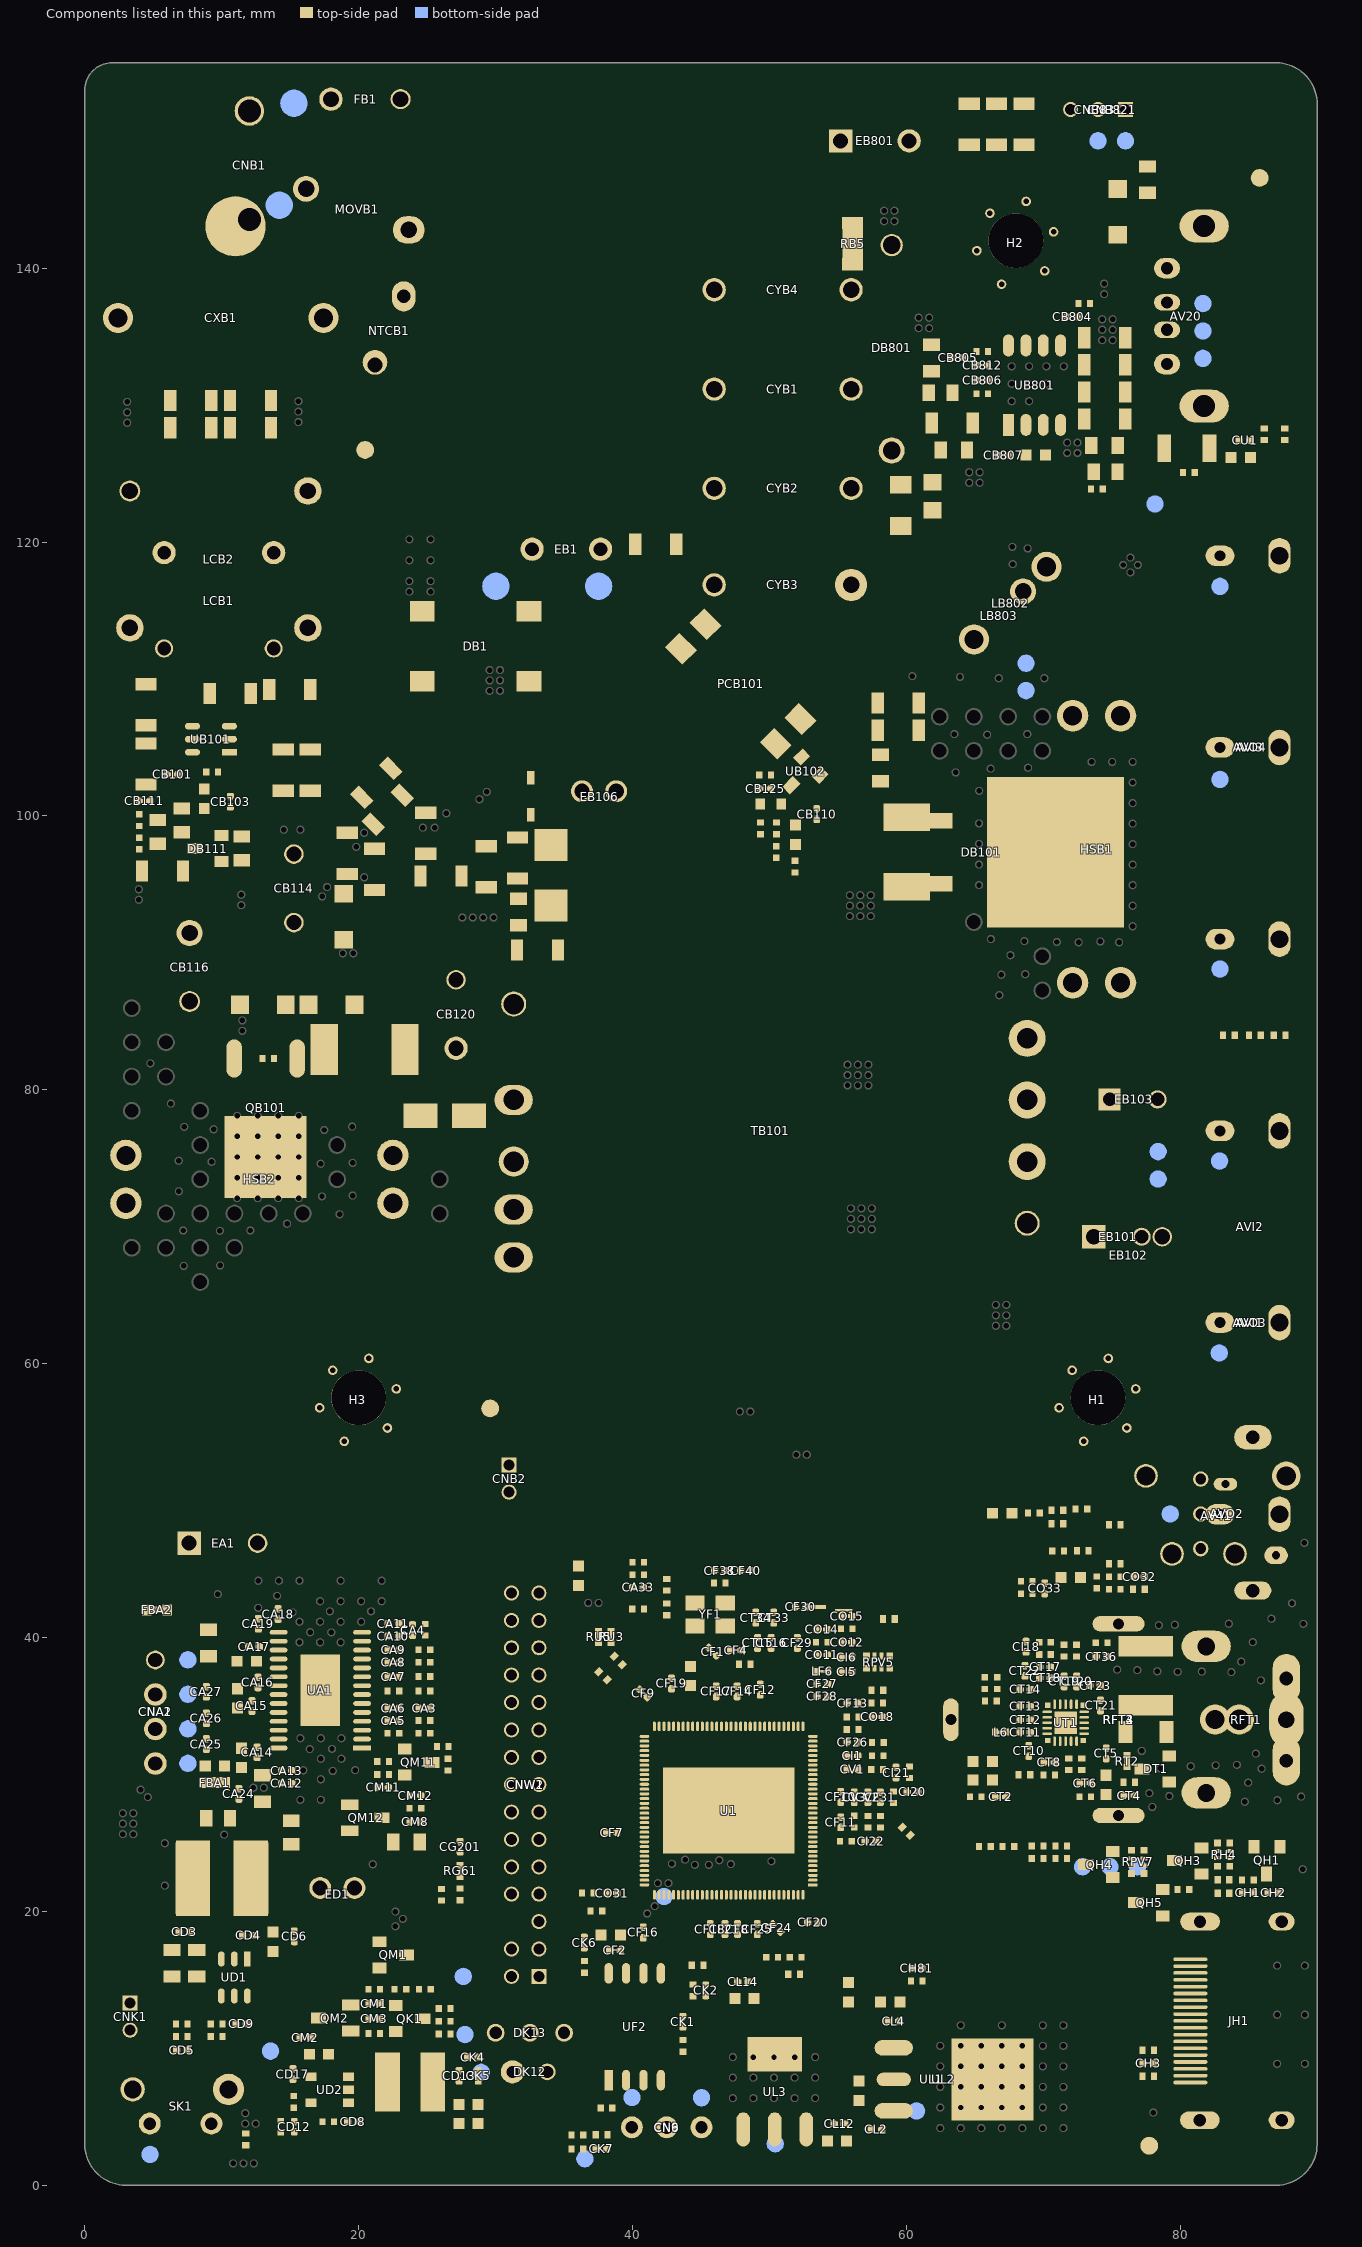
[diagram p0: the components of this part, seen from the top]
# Altium PCB MISC116569.PcbDoc (part 14 of 15)
Units mm, origin at the board's own origin, x right, y up, seen from the top; angles counter-clockwise.
Board outline 90 x 155 mm, 2 copper layers (TopLayer, BottomLayer), stack 1.571 mm thick; 527 components, 277 nets, 2450 pads, 649 vias.

## Other copper (continued)
BottomLayer:
  rectangle net GND: 77.495,141.897 84.887,146.863
  rectangle net GND: 75.908,22.327 77.787,24.257
  rectangle net D_QB101: 20.498,72.034 25.019,78.245
  rectangle net D_QB101: 0.902,69.113 5.927,80.124
  rectangle net 12V: 69.413,103.543 76.716,109.715
  rectangle net 12V: 68.982,87.77 76.665,93.154
  rectangle net 12V: 63.279,86.309 69.731,91.135
  rectangle net GND: 29.853,38.367 34.425,40.361
  rectangle net GND: 32.063,18.542 34.615,20.17
  rectangle net GND: 29.154,26.264 35.644,28.308
  rectangle net GND: 87.219,32.182 89.365,38.024
  rectangle net GND: 61.692,31.394 66.099,36.208
  rectangle net GND: 72.766,38.964 78.113,42.469
  rectangle net GND: 79.269,37.287 84.945,41.427
  rectangle net GND: 85.784,28.74 89.175,40.424
  rectangle net GND: 79.459,26.873 84.933,31.013
  rectangle: 288.542,50.641 291.849,52.641
  rectangle net GND: 78.334,129.184 86.436,130.797
  rectangle net GND: 81.039,127.343 82.41,131.801
  rectangle net 12V: 67.386,107.366 70.371,112.738
  rectangle net 12V: 62.941,110.795 66.7,114.465
  rectangle net GND: 39.484,31.877 41.491,34.341
  pour cut-out: 85.124,51.2 85.124,47.21 84.772,47.561 83.833,47.561 83.833,49.073 83.617,49.289 83.617,50.419
  pour cut-out: 81.955,116.786 81.955,117.337 81.581,117.711 81.644,117.774 82.323,117.774 82.705,117.392 82.676,117.364 82.676,117.095
  pour cut-out: 83.848,116.767 83.848,117.274 84.361,117.787 84.316,117.831 82.925,117.831 82.925,117.069 83.268,116.726 83.337,116.726
  pour cut-out: 81.955,102.688 81.955,103.366 81.55,103.772 82.228,103.772 82.705,103.295 82.677,103.266 82.677,102.997
  pour cut-out: 83.849,102.669 83.849,103.176 84.362,103.689 84.317,103.734 82.925,103.734 82.925,102.972 83.268,102.629 83.337,102.629
  pour cut-out: 81.955,88.833 81.955,89.384 81.581,89.758 81.644,89.822 82.323,89.822 82.705,89.44 82.676,89.411 82.676,89.142
  pour cut-out: 83.848,88.814 83.848,89.321 84.361,89.834 84.316,89.879 82.925,89.879 82.925,89.117 83.268,88.774 83.337,88.774
  pour cut-out: 81.904,60.804 81.904,61.355 81.531,61.729 81.594,61.792 82.273,61.792 82.655,61.41 82.626,61.382 82.626,61.112
  pour cut-out: 83.798,60.785 83.798,61.291 84.311,61.804 84.266,61.849 82.875,61.849 82.875,61.087 83.217,60.744 83.287,60.744
  pour cut-out: 83.823,74.793 83.823,75.299 84.336,75.812 84.292,75.857 82.9,75.857 82.9,75.095 83.243,74.752 83.312,74.752
  pour cut-out: 81.93,74.812 81.93,75.363 81.556,75.737 81.619,75.8 82.298,75.8 82.68,75.418 82.652,75.39 82.652,75.12
  region net N-2: 15.311,146.037 11.366,146.037 10.071,144.742 10.071,144.069 11.862,142.278 14.453,144.869 15.011,144.869 15.011,145.422 15.387,145.797
  region net NetDB109_A: 3.759,94.932 3.632,94.805 3.632,93.599 3.95,93.281 4.255,93.586 4.255,94.767 4.089,94.932
  region net D_QB101: 18.796,90.361 18.542,90.106 18.542,89.065 19.266,88.341 20.015,89.09 20.015,90.157 19.812,90.361
  region net VBRIDGE: 29.019,119.685 29.82,120.485 32.067,120.485 32.969,119.583 32.093,119.583 30.886,118.377 30.886,112.357 29.959,111.43 29.019,112.37
  region net L-5: 23.254,138.303 24.168,138.303 27.173,141.308 27.173,140.246 29.472,137.947 24.574,137.947
  region net GND: 87.008,58.001 82.956,58.001 81.928,56.972 81.928,54.661 83.655,52.934 86.55,52.934 86.55,53.01 88.062,54.521 88.062,57.379
  region net D_QB101: 16.205,78.067 17.335,78.067 19.52,80.251 22.466,77.305 20.764,77.305 19.901,76.441
  region net SNB-RM: 21.73,99.416 19.787,99.416 19.52,99.149 19.52,97.447 19.774,97.193 22.218,97.193 22.377,97.353 22.377,98.768
  pour cut-out: 50.076,68.123 62.179,68.123 63.983,66.319 63.327,65.664 52.301,65.664 49.949,68.016
  region net GND: 62.357,137.706 62.357,128.003 64.008,126.352 64.351,126.352 64.351,127.419 67.107,130.175 64.16,133.121 63.83,133.121 63.83,135.369 64.414,135.953 62.789,137.579 62.789,137.808
  region net EPH_DET_IN/GND: 81.978,52.134 82.271,51.841 83.045,51.841 83.134,51.752 83.134,50.787 82.906,50.559 81.991,50.559 81.229,51.321 81.229,51.397
  region net GND: 15.634,58.45 15.634,54.254 10.592,49.212 19.164,49.212 19.533,49.581 23.99,49.581 24.009,49.6 17.539,56.07 17.539,58.604
  pour cut-out: 65.951,62.268 61.417,66.802 66.357,66.802 68.923,64.237 66.954,62.268
  pour cut-out: 52.301,65.2 43.661,65.2 44.247,65.786 44.247,69.977 48.814,69.977 49.22,70.383
  pour cut-out: 59.333,24.405 59.103,24.176 58.656,24.176 58.656,23.94 58.49,23.773 58.922,23.773 58.924,23.771
  pour cut-out: 63.513,24.451 62.956,24.451 62.862,24.546 62.862,23.639 62.817,23.594
  pour cut-out: 60.376,23.803 60.315,23.803 59.807,24.311 59.778,24.282 59.778,23.62 60.03,23.368 60.376,23.368
  pour cut-out: 56.494,14.174 55.731,14.174 55.299,13.742 55.299,14.24 56.401,15.342 56.443,15.342
  region net GND: 85.136,44.688 84.19,43.743 83.427,43.743 82.281,42.596 81.039,42.596 83.134,40.5 87.922,40.5 87.922,44.463 88.303,44.844 87.605,45.542 86.487,45.542 85.623,44.679 85.145,44.679
  region net GND: 213 vertices and 0 holes, not listed, extent 30.47,52.61 31.506,54.486
  pour cut-out: 25.826,58.585 25.078,58.585 23.364,60.298 23.364,60.867 24.363,60.867 25.26,59.969 26.152,59.969
  pour cut-out: 15.612,59.32 15.612,57.319 15.049,56.756 14.91,56.896 14.199,56.896 14.199,59.22 14.148,59.271
  region net D_QB101: 8.077,87.389 8.534,86.931 8.534,83.401 7.671,82.537 6.502,83.706 5.169,83.706 5.169,83.896 4.547,84.519 4.547,86.601 5.334,87.389
  region net 5V_M: 12.784,4.75 12.784,5.423 12.644,5.563 11.578,5.563 11.412,5.397 11.412,4.242 11.806,3.848 11.92,3.962 12.149,3.962
  region net 5V_M: 12.784,3.124 12.784,1.486 12.581,1.283 10.676,1.283 10.511,1.448 10.511,1.968 11.793,3.251 12.149,3.251
  region net GND: 63.432,125.692 65.413,125.692 65.781,125.324 65.781,124.015 65.641,123.876 63.775,123.876 62.657,124.993 62.835,125.171 62.835,125.235
  region net L: 12.784,114.22 12.784,112.039 13.432,111.392 15.362,111.392 17.343,113.373 17.343,114.808 16.835,114.3 12.864,114.3
  region net N-2: 1.456,124.93 1.456,120.536 3.386,118.605 6.447,118.605 6.51,118.542 6.802,118.834 6.802,120.222 2.431,124.593
  region net L: 15.074,114.269 14.492,115.971 13.941,114.269
  region net L: 16.192,114.269 15.609,115.971 15.058,114.269
  region net L: 13.966,114.269 13.384,115.971 12.833,114.269
  region net N-2: 5.537,118.726 6.12,117.023 6.671,118.726
  region net N-2: 3.312,118.726 3.894,117.023 4.445,118.726
  region net N-2: 4.43,118.726 5.012,117.023 5.563,118.726
  region net L-1: 18.372,154.47 18.817,154.026 18.817,150.952 18.296,150.431 11.743,150.431 11.717,150.457 11.717,152.883 13.305,154.47
  region net GND: 76.848,81.547 76.848,77.826 75.908,76.886 69.063,76.886 68.097,75.921 68.097,73.685 68.986,72.796 75.768,72.796 77.406,71.158 78.6,72.352 78.6,73.952 78.829,74.181 78.283,74.727 78.283,81.547
  pour cut-out: 36.076,46.151 36.432,46.151 36.755,45.828 37.054,46.126 37.054,46.698 36.876,46.876
  pour cut-out: 35.572,47.448 35.572,46.654 35.64,46.586 35.68,46.626 36.116,46.626 36.116,46.801 36.528,47.212
  pour cut-out: 40.787,46.29 40.216,46.29 40.032,46.107 39.771,46.368 39.771,46.734 39.568,46.937
  pour cut-out: 41.214,47.699 41.214,46.734 41.012,46.937 40.576,46.937 40.576,47.366 40.421,47.522
  pour cut-out: 52.916,17.123 52.916,15.946 52.783,15.813 52.951,15.645 53.085,15.779 53.085,16.241 53.659,16.815
  region net GND: 72.601,30.099 77.351,30.099 78.735,28.715 77.694,27.673 77.694,26.683 77.592,26.581 77.592,26.06 76.69,25.159 73.858,25.159 71.115,27.902 70.81,27.902 70.81,29.451 72.08,30.721 72.347,30.721
  region net VCC_PANEL: 24.125,17.12 24.125,19.317 23.16,20.282 22.525,20.282 22.385,20.142 22.385,18.212 23.287,17.31 23.496,17.31
  region net 3V3_STB: 64.524,13.261 72.779,13.261 75.446,10.594 75.446,1.869 75.014,1.438 60.066,1.438 59.19,2.314 59.19,7.927
  region net +1.8V_DDR: 47.29,10.366 46.507,9.583 46.507,3.251 47.623,2.136 53.322,2.136 54.249,3.063 54.249,9.413 53.297,10.366
  region net VDDC_CORE: 42.794,22.354 41.613,22.354 41.524,22.266 41.524,21.135 40.762,20.373 40.762,19.599 40.94,19.421 41.473,19.421 42.959,20.907 42.959,22.189
  region net GND: 213 vertices and 0 holes, not listed, extent 2.792,13.319 3.828,15.196
  region net VDDC_CORE: 39.086,41.392 37.651,42.827 36.622,42.827 36.457,42.662 36.457,42.395 38.476,40.376 42.883,40.376 43.048,40.541 43.048,41.239 42.896,41.392
  region net GND: 60.206,149.962 59.372,149.962 58.052,148.641 58.052,143.281 58.204,143.129 59.868,143.129 60.117,143.378 60.117,147.917 60.193,147.993 60.737,147.993 60.865,148.122 60.865,149.302
  region net VBRIDGE: 29.019,115.139 29.019,113.373 26.733,111.087 26.733,109.309 27.241,108.801 30.34,108.801 30.886,109.347 30.886,115.392 29.908,116.37
  region net N-3: 25.895,124.841 25.895,114.859 24.27,113.233 23.597,113.233 23.431,113.398 23.431,123.876 24.892,125.336 25.189,125.04 25.997,125.04
  region net NetDB109_A: 10.77,86.68 10.77,84.074 10.846,83.998 11.646,83.998 11.811,84.163 11.811,85.636 10.907,86.54 10.907,86.553
  region net L-2: 12.812,118.573 12.812,119.662 14.219,121.069 15.087,121.069 16.16,119.996 16.16,118.573 16.129,118.542 12.843,118.542
  region net L-2: 15.027,118.573 15.609,116.871 16.16,118.573
  region net L-2: 13.919,118.573 14.502,116.871 15.053,118.573
  region net L-2: 12.812,118.573 13.394,116.871 13.945,118.573
  pour cut-out: 62.192,136.385 64.643,133.934 75.87,133.934 75.844,134.01 75.565,134.29 64.96,134.29 62.192,137.058
  pour cut-out: 75.87,133.934 75.87,138.76 75.768,138.862 75.578,138.862 75.413,138.697 75.413,134.645 74.854,134.087 74.689,134.087 74.803,133.972 75.857,133.972
  region net SGND: 28.429,94.075 27.267,92.913 27.267,92.378 27.368,92.277 30.074,92.277 30.162,92.365 30.162,92.785 29.769,93.178 29.769,94.245 29.654,94.245 29.604,94.296
  region net VBRIDGE: 24.384,93.841 24.384,100.368 24.714,100.698 27.559,100.698 28.6,101.74 29.159,101.181 29.159,99.276 25.336,95.453 25.336,94.678
  region net GND: 63.932,134.645 63.932,134.874 64.821,135.763 62.509,138.074 62.395,138.074 62.873,137.597 62.873,133.037 64.198,131.712 64.364,131.877 64.77,131.877 64.77,133.807
  region net DRIM: 73.825,130.848 70.955,130.848 70.294,130.188 70.294,125.298 66.827,121.831 66.827,116.154 67.513,115.468 71.945,115.468 74.193,117.716 74.193,130.48
  pour cut-out: 63.132,150.419 76.492,150.419 78.956,147.955 76.289,147.955 74.13,145.796 74.13,139.205 73.377,139.205 73.035,138.863 73.035,144.541 70.396,147.18 65.799,147.18 64.897,146.279 63.36,147.815 63.36,149.352 62.916,149.796
  pour cut-out: 72.191,144.315 72.787,143.719 72.787,142.004 73.399,142.004 73.546,142.151 73.495,142.202 73.495,146.202 73.165,146.202 72.923,146.444
  region net GND: 77.495,146.863 67.018,146.863 66.319,146.164 68.707,146.164 71.006,143.866 71.006,139.789 72.123,140.906 74.429,140.906 76.187,139.148 76.493,139.454 80.25,139.454 80.282,139.487 86.312,139.487 87.414,140.589 87.414,141.999 88.049,142.634 86.208,144.475 79.883,144.475
  pour cut-out: 16.256,55.736 16.256,50.317 3.708,50.317 -0.254,46.355 -0.254,45.161 -0.483,45.161 -0.483,59.957 2.222,62.662 18.834,62.662 19.431,63.259 19.431,62.56 17.094,60.223 16.739,60.223 15.862,59.347 15.862,56.13
  pour cut-out: 16.256,50.317 18.012,52.074 18.012,53.98 16.798,55.194 14.491,55.194 14.491,54.356 13.995,53.861 14.389,53.467 14.389,52.768
  region net GND: 24.109,59.739 25.264,58.585 39.56,58.585 42.583,55.562 38.697,51.676 27.851,51.676 23.381,56.147 23.381,59.13 23.99,59.739
  pour cut-out: 31.164,26.011 33.164,26.011 32.893,25.74 32.893,25.375 32.047,25.375 31.923,25.251 31.686,25.489 31.305,25.489
  pour cut-out: 29.738,24.707 30.43,25.399 30.43,25.448 30.534,25.448 31.242,24.74 30.775,24.272 30.493,24.272
  pour cut-out: 34.463,25.203 34.266,25.203 33.769,25.7 33.172,25.104 33.172,24.501 33.401,24.272 33.968,24.272
  pour cut-out: 29.738,23.837 29.819,23.837 30.404,23.251 30.698,23.546 31.229,23.546 31.229,24.044 31.001,24.272
  pour cut-out: 31.544,22.594 33.062,22.594 32.842,22.813 32.842,23.609
  pour cut-out: 33.923,23.251 33.923,23.77 34.491,24.338 34.233,24.596 33.829,24.596 33.058,23.825
  pour cut-out: 30.522,18.594 30.366,18.438 30.366,17.935 30.171,17.935 29.98,17.744 29.544,18.18 29.522,18.18
  region net GND: 45.975,6.5 46.127,6.349 46.127,10.211 45.314,9.398 44.983,9.398 45.949,8.433 45.949,7.074 45.987,7.036 45.987,6.528
  region net GND: 45.966,3.626 46.127,3.786 46.127,3.162 46.914,2.375 46.914,2.146 46.849,2.081 45.785,2.081 45.555,2.311 45.555,2.388 45.966,2.799
  pour cut-out: 25.844,58.585 25.387,58.585 24.066,59.906 24.066,60.515 24.638,61.087 24.994,60.731 25.59,60.731 25.59,59.207 25.908,58.89
  region net 12V: 8.788,29.197 3.937,29.197 3.772,29.032 3.772,28.067 3.95,27.889 8.674,27.889 9.461,28.677 9.385,28.753 9.385,29.096
  region net 12V: 2.324,30.493 2.324,28.943 3.861,27.407 3.861,25.413 3.594,25.146 1.346,25.146 0.889,25.603 0.889,29.121 1.257,29.489
  region net SNB-D-: 15.469,91.326 17.526,93.383 21.311,93.383 21.399,93.472 21.399,95.479 21.018,95.86 18.186,95.86 14.813,92.486 14.813,92.477 14.701,92.365
  pour cut-out: 74.13,139.205 74.905,139.205 76.111,137.998 76.429,137.998 76.429,138.9 75.286,140.043 73.765,140.043
  pour cut-out: 59.398,67.539 70.104,67.539 70.548,67.094 67.094,63.64 67.094,63.208 66.624,63.208 66.497,63.335 66.497,64.122 65.43,65.189 61.232,65.189 59.238,67.183 58.572,67.183
  region net NetCB114_1: 13.982,99.338 12.954,98.311 12.954,96.901 13.538,96.317 15.621,96.317 16.015,96.71 16.015,96.89 17.411,98.287 17.411,98.59 16.664,99.338
  region net GND: 76.187,139.141 75.286,140.043 74.13,140.043 73.266,140.906 72.559,140.906 72.356,141.11 72.356,143.171 76.094,143.171 77.203,142.062 77.203,136.055 76.2,137.058 76.2,137.122 76.187,137.135
  pour cut-out: 76.454,118.618 77.991,118.618 79.17,119.797 79.17,118.669 78.499,117.997 78.499,117.043 77.978,117.043 77.914,116.98
  pour cut-out: 78.347,48.824 78.347,47.58 77.922,47.155 78.633,46.444 79.083,46.444 79.997,47.358
  pour cut-out: 79.807,52.743 79.921,52.629 79.921,50.838 79.023,49.94 79.939,49.024 81.359,49.024 81.813,49.479 81.813,52.158 81.2,52.772
  pour cut-out: 82.273,53.177 82.273,52.855 82.906,52.222 82.906,51.994 82.601,51.994 82.398,51.791 82.017,52.172 81.559,52.172
  pour cut-out: 80.235,43.743 79.337,44.64 80.759,46.063 80.759,46.774 83.326,46.774 84.19,45.91 84.252,45.91 84.252,44.056 84.366,43.942 84.167,43.743
  region net GND: 68.986,72.796 74.333,72.796 75.108,72.022 75.108,68.326 73.894,67.113 73.615,67.113 73.615,66.39 74.524,65.481 76.073,67.031 76.073,67.107 80.886,67.107 81.077,67.297 79.21,69.164 79.21,74.32 75.946,74.32 74.866,75.4 69.583,75.4 68.986,74.803
  region net EPH_LOUT/COAX: 79.629,47.092 83.96,47.092 84.176,46.876 84.176,45.441 83.833,45.098 79.388,45.098 78.93,45.555 78.93,45.885
  region net 12V: 76.995,87.536 75.959,86.5 75.959,86.497 74.196,84.734 71.615,84.734 69.532,86.817 69.647,86.931 69.647,88.938 72.403,91.694 74.803,91.694 76.995,89.502
  region net 12V: 76.995,112.662 76.995,105.532 76.035,104.572 74.371,106.236 72.098,106.236 72.098,107.404 71.996,107.505 71.996,107.663
  region net GND: 63.023,65.126 66.173,61.976 70.231,61.976 64.071,55.816 59.88,55.816 57.353,58.344 58.318,59.309 58.318,63.678 59.766,65.126
  pour cut-out: 82.556,117.868 ccw(c82.9,116.767) 84.053,116.767 ccw(c82.9,116.767) 83.5,117.752 ccw(c83.37,117.538) 83.24,117.324 cw(c82.9,116.767) 83.552,116.767 cw(c82.9,116.767) 82.705,117.39 ccw(c82.631,117.629) 82.881,117.629 ccw(c82.631,117.629)
  pour cut-out: 82.557,103.77 ccw(c82.901,102.669) 84.054,102.669 ccw(c82.901,102.669) 83.501,103.654 ccw(c83.371,103.44) 83.24,103.226 cw(c82.901,102.669) 83.553,102.669 cw(c82.901,102.669) 82.706,103.292 ccw(c82.632,103.531) 82.882,103.531 ccw(c82.632,103.531)
  pour cut-out: 82.556,89.915 ccw(c82.9,88.814) 84.053,88.814 ccw(c82.9,88.814) 83.5,89.799 ccw(c83.37,89.585) 83.24,89.371 cw(c82.9,88.814) 83.552,88.814 cw(c82.9,88.814) 82.705,89.437 ccw(c82.631,89.676) 82.881,89.676 ccw(c82.631,89.676)
  pour cut-out: 82.506,61.885 ccw(c82.85,60.785) 84.003,60.785 ccw(c82.85,60.785) 83.45,61.769 ccw(c83.32,61.556) 83.189,61.342 cw(c82.85,60.785) 83.502,60.785 cw(c82.85,60.785) 82.655,61.407 ccw(c82.581,61.646) 82.831,61.646 ccw(c82.581,61.646)
  pour cut-out: 82.531,75.894 ccw(c82.875,74.793) 84.029,74.793 ccw(c82.875,74.793) 83.475,75.778 ccw(c83.345,75.564) 83.215,75.35 cw(c82.875,74.793) 83.528,74.793 cw(c82.875,74.793) 82.681,75.416 ccw(c82.606,75.655) 82.856,75.655 ccw(c82.606,75.655)
  pour cut-out: 70.711,83.75 cw(c68.814,83.75) 70.262,84.977 cw(c70.071,84.815) 70.321,84.815 cw(c70.071,84.815) 69.88,84.653 ccw(c68.814,83.75) 70.211,83.75 ccw(c68.814,83.75) 70.157,84.133 cw(c70.398,84.201) 70.639,84.27 cw(c68.814,83.75)
  pour cut-out: 66.918,83.71 ccw(c67.168,83.716) 67.419,83.716 ccw(c67.168,83.716) 67.419,83.721 cw(c68.814,83.75) 70.211,83.75 cw(c68.814,83.75) 70.21,83.723 ccw(c70.461,83.718) 70.711,83.713 ccw(c68.814,83.75) 70.711,83.75 ccw(c68.814,83.75)
  pour cut-out: 73.794,142.004 cw(c68,142.004) 72.994,144.94 cw(c72.556,144.683) 73.065,144.683 cw(c72.556,144.683) 72.118,144.425 ccw(c68,142.004) 72.777,142.004 ccw(c68,142.004) 72.775,142.153 cw(c73.283,142.169) 73.791,142.184 cw(c68,142.004)
  pour cut-out: 80.25,139.454 82.084,139.454 cw(c82.084,138.43) 83.109,138.43 83.109,132.118 cw(c82.88,132.118) 82.88,131.889 79.184,131.889 cw(c79.184,133.121) 77.953,133.121 77.953,133.871 cw(c78.168,133.871) 78.168,134.087
  pour cut-out: 17.215,53.668 ccw(c17.514,54.079) 18.022,54.079 ccw(c17.514,54.079) 17.812,54.49 cw(c20,57.502) 23.16,59.471 ccw(c23.591,59.739) 24.099,59.739 ccw(c23.591,59.739) 24.023,60.008 ccw(c20,57.502)
  text ".GBL" at 303.152,51.191 h1.52
  text "BottomLayer" at 292.423,51.153 h1.52

## Silkscreen, mask and mechanical layers (free items; w line width, h text height)
TopOverlay:
  drawing of 523 lines, arcs and shapes, not listed
  text "3" at 94.89,240.834 h4.06 r180
  text "4" at 85.119,224.173 h4.06
  text "Solder Mask:" at 285.116,182.17 h1.52
  text "IPC SM-840" at 295.593,182.144 h1.52
  text "Silkscreen Color:" at 315.049,182.144 h1.52
  text "White" at 327.216,182.144 h1.52
  text "Units:" at 315.049,179.63 h1.52
  text "PTH Copper Thickness:" at 285.116,179.604 h1.52
  text "mm" at 320.079,179.592 h1.52
  text ">20um" at 302.222,179.579 h1.52
  text "4.2 --- 4.6" at 315.066,177.103 h1.52
  text "Dielectric Constant Er@1GHz To 1MHz:" at 285.107,177.09 h1.52
  text "Panel Size:" at 285.065,174.588 h1.52
  text "2L,4,90.00×155.00mm,FR4(TG130-CTI175),1OZ,Green,OSP,1.6mm" at 292.816,174.588 h1.52
  text "Silkscreen on PTH:" at 285.077,172.01 h1.52
  text "Primary Side Retained;" at 298.235,171.984 h1.52
  text "Secondary Side  Removed for Soldering" at 315.049,171.946 h1.52
  text "Special Requirements" at 285.052,169.706 h1.52
  text "No reply within 2 hours on engineering questions; call PHONE_A" at 332.973,169.521 h1.52
  text "1. Lead-free hot air solder leveling (HAL_LF, Lead Free Hot Air Leveling)" at 300.06,167.075 h1.52
  text "2. Organic solderability preservative (OSP, Organic Solderability Preservatives)" at 300.06,164.942 h1.52
  text "3. Electroless nickel/immersion gold (ENIG, Electroless Nickel/Immersion Gold)" at 300.022,162.618 h1.52
  text "Plated Technics" at 286.957,161.735 h1.52
  text "4. Electroless nickel/immersion gold + gold finger (ENIG_G/F, Electroless Nickel/Immersion Gold + Gold Finger)" at 300.06,160.573 h1.52
  text "5. Gold plating (Gold_plated, Gold-plated)" at 300.086,158.528 h1.52
  text "6. Gold plating + gold finger (Gold_Plated_G/F, Gold-plated + Gold Finger)" at 300.099,156.547 h1.52
  text "Impedance Control" at 285.172,150.741 h1.52
  text "Target Impedance" at 305.412,150.743 h1.52
  text "Width & Clearance" at 324.356,150.737 h1.52
  text "Layer(s)" at 343.871,150.745 h1.52
  text "LED DRIVER" at 78.702,148.755 h1.52
  text "75 +/- 10% Ohm" at 305.976,148.185 h1.52
  text "G/12/15.8/12/G mil" at 323.274,148.168 h1.52
  text "layer 1" at 343.871,148.171 h1.52
  text "Single End Impedance" at 285.172,147.011 h1.52
  text "[ Zo ]" at 290.849,143.525 h1.52
  text "G/5/7/5/7/5/G mil" at 323.528,138.237 h1.52
  text "100 +/- 10% Ohm" at 305.646,138.211 h1.52
  text "layer 1" at 344.15,138.166 h1.52
  text "Differential Impedance" at 285.169,136.811 h1.52
  text "[ Zo ]" at 290.836,133.679 h1.52
  text "( G: Ground )" at 288.552,130.948 h1.52
  text "90 +/- 10% Ohm" at 306.307,130.642 h1.52
  text "layer 1" at 344.049,130.622 h1.52
  text "G/5/11/5/11/5/G mil" at 323.528,130.553 h1.52
  text "Common Mode Impedance" at 284.655,125.317 h1.52
  text "[ Zc ]" at 290.954,123.26 h1.52
  text "Refer to Gerber documents GTP&GBP for Stencil aperture design" at 307.898,116.55 h1.52
  text "Stencil (Stencil)" at 285.018,114.086 h1.52
  text "New" at 307.844,111.608 h1.52
  text "Testing jig (Testing jig)" at 284.97,109.116 h1.52
  text "New" at 307.844,109.061 h1.52
  text "Wave-soldering jig (Wave-soldering jig)" at 285.026,106.621 h1.52
  text "New" at 307.844,106.518 h1.52
  text "Production process (Production process)" at 284.987,103.998 h1.52
  text "Solder paste" at 307.81,102.883 h1.52
  text "SMD components are 3.5mm from the PCB edge; special production control required" at 316.928,102.616 h1.52
  text "[Process and precautions]" at 289.565,101.843 h1.52
  text "HDMI (FB1离VCUT边太近分板时参考HDMI分板方式）;EB801需MI" at 307.886,98.988 h1.27
  text "Special requirements (Special Requirements)" at 285.013,98.968 h1.52
  text "SMD components over 2mm high on the solder side (wave soldering)" at 285.005,96.394 h1.52
  text "Package attention (Package Attention)" at 284.997,93.951 h1.52
  text "[Easily damaged components]" at 291.127,91.797 h1.52
  text "Footprint matching (Footprint Matching)" at 284.997,88.871 h1.52
  text "[New component footprint]" at 290.771,86.742 h1.52
  text "2" at 94.89,85.832 h4.06 r180
  text "(Automated Testing Support)" at 293.083,83.834 h1.14
  text "Automated testing support" at 284.993,83.745 h1.52
  text "[Reserved suction cup and press bar positions]" at 289.069,81.599 h1.52
  text "Layer Stack Up Detail for" at 288.577,72.467 h2.54
  text ".Pcb_File_Name_No_Path" at 315.522,72.467 h2.54
  text "1" at 85.119,69.171 h4.06
  text "Layer" at 292.751,68.715 h1.27
  text "Gerber" at 302.193,68.715 h1.27
  text "Layer" at 310.096,68.715 h1.27
  text "Layer" at 326.257,68.715 h1.27
  text "Copper" at 346.295,68.715 h1.27
  text "Dielectric" at 354.214,68.715 h1.27
  text "Stack up" at 326.257,67.422 h1.27
  text "Height" at 354.214,67.422 h1.27
  text "Name" at 292.751,67.384 h1.27
  text "Document" at 302.193,67.384 h1.27
  text "Ordor" at 310.096,67.384 h1.27
  text "Thickness" at 346.295,67.384 h1.27
  text "TopOverlay" at 292.744,61.47 h1.52
  text ".GTO" at 303.147,61.405 h1.52
  text "0.4mil" at 354.146,59.245 h1.52
  text "1" at 311.447,56.625 h1.52
  text "1.4mil" at 346.626,56.623 h1.52
  text "GND" at 33.311,52.235 h1.27
  text "2" at 311.449,51.214 h1.52
  text "1.4mil" at 346.583,51.188 h1.52
  text "12V" at 33.311,50.235 h1.27
  text "0.4mil" at 354.214,48.783 h1.52
  text "PWR UPGRADE" at 25.936,46.828 h1.52
  text "BOE" at 50.317,44.386 h5
  text "SPEAKER" at 2.045,41.618 h1.52 r90
  text "LVDS" at 37.567,27.254 h1.52 r90
  text "KEY" at 0.686,15.888 h1.52
  text "LED" at 24.244,1.321 h1.52
  text "KEY" at 12.687,1.092 h1.52
  text "IR" at 48.438,0.521 h1.52